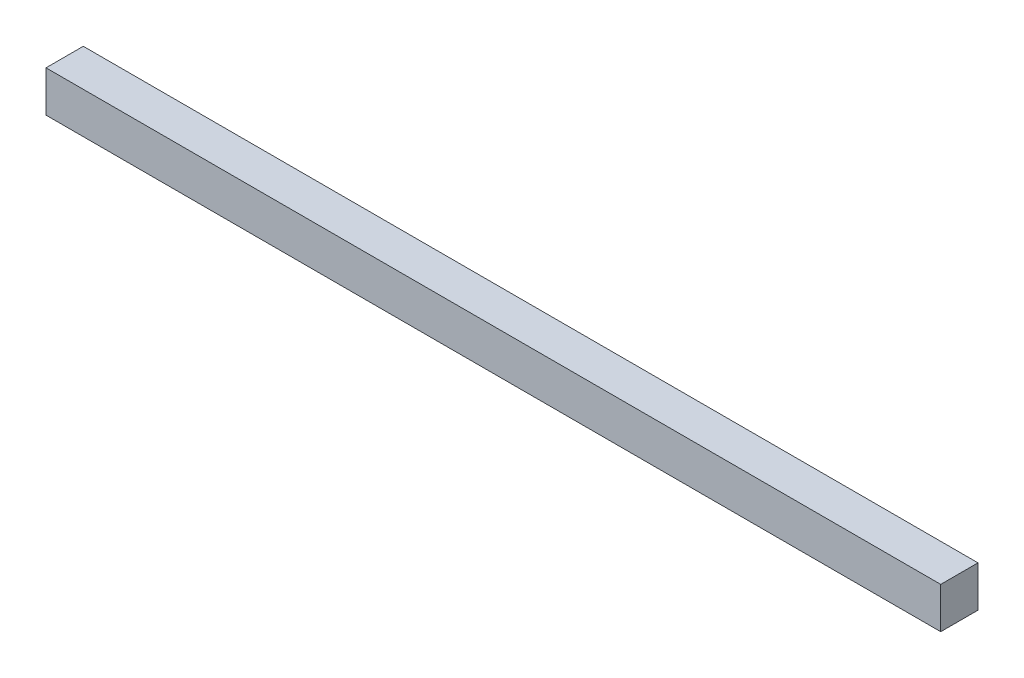
SolidWorks part; units mm, degrees
material "Q235B"
ref_plane "Front Plane" through (0, 0, 0) normal (0, 0, 1) x (1, 0, 0)
ref_plane "Top Plane" through (0, 0, 0) normal (0, 1, 0) x (1, 0, 0)
ref_plane "Right Plane" through (0, 0, 0) normal (1, 0, 0) x (0, 0, -1)
sketch "Sketch1" plane through (0, 0, 0) normal (0, 0, 1) x (1, 0, 0)
  line L1 (0, 0) -> (480, 0)
  line L2 (0, 0) -> (0, 22)
  line L3 (0, 22) -> (480, 22)
  line L4 (480, 0) -> (480, 22)
  dimension "D1" = 480
  dimension "D2" = 22
extrude "Boss-Extrude1" add sketch "Sketch1" along normal blind 20
